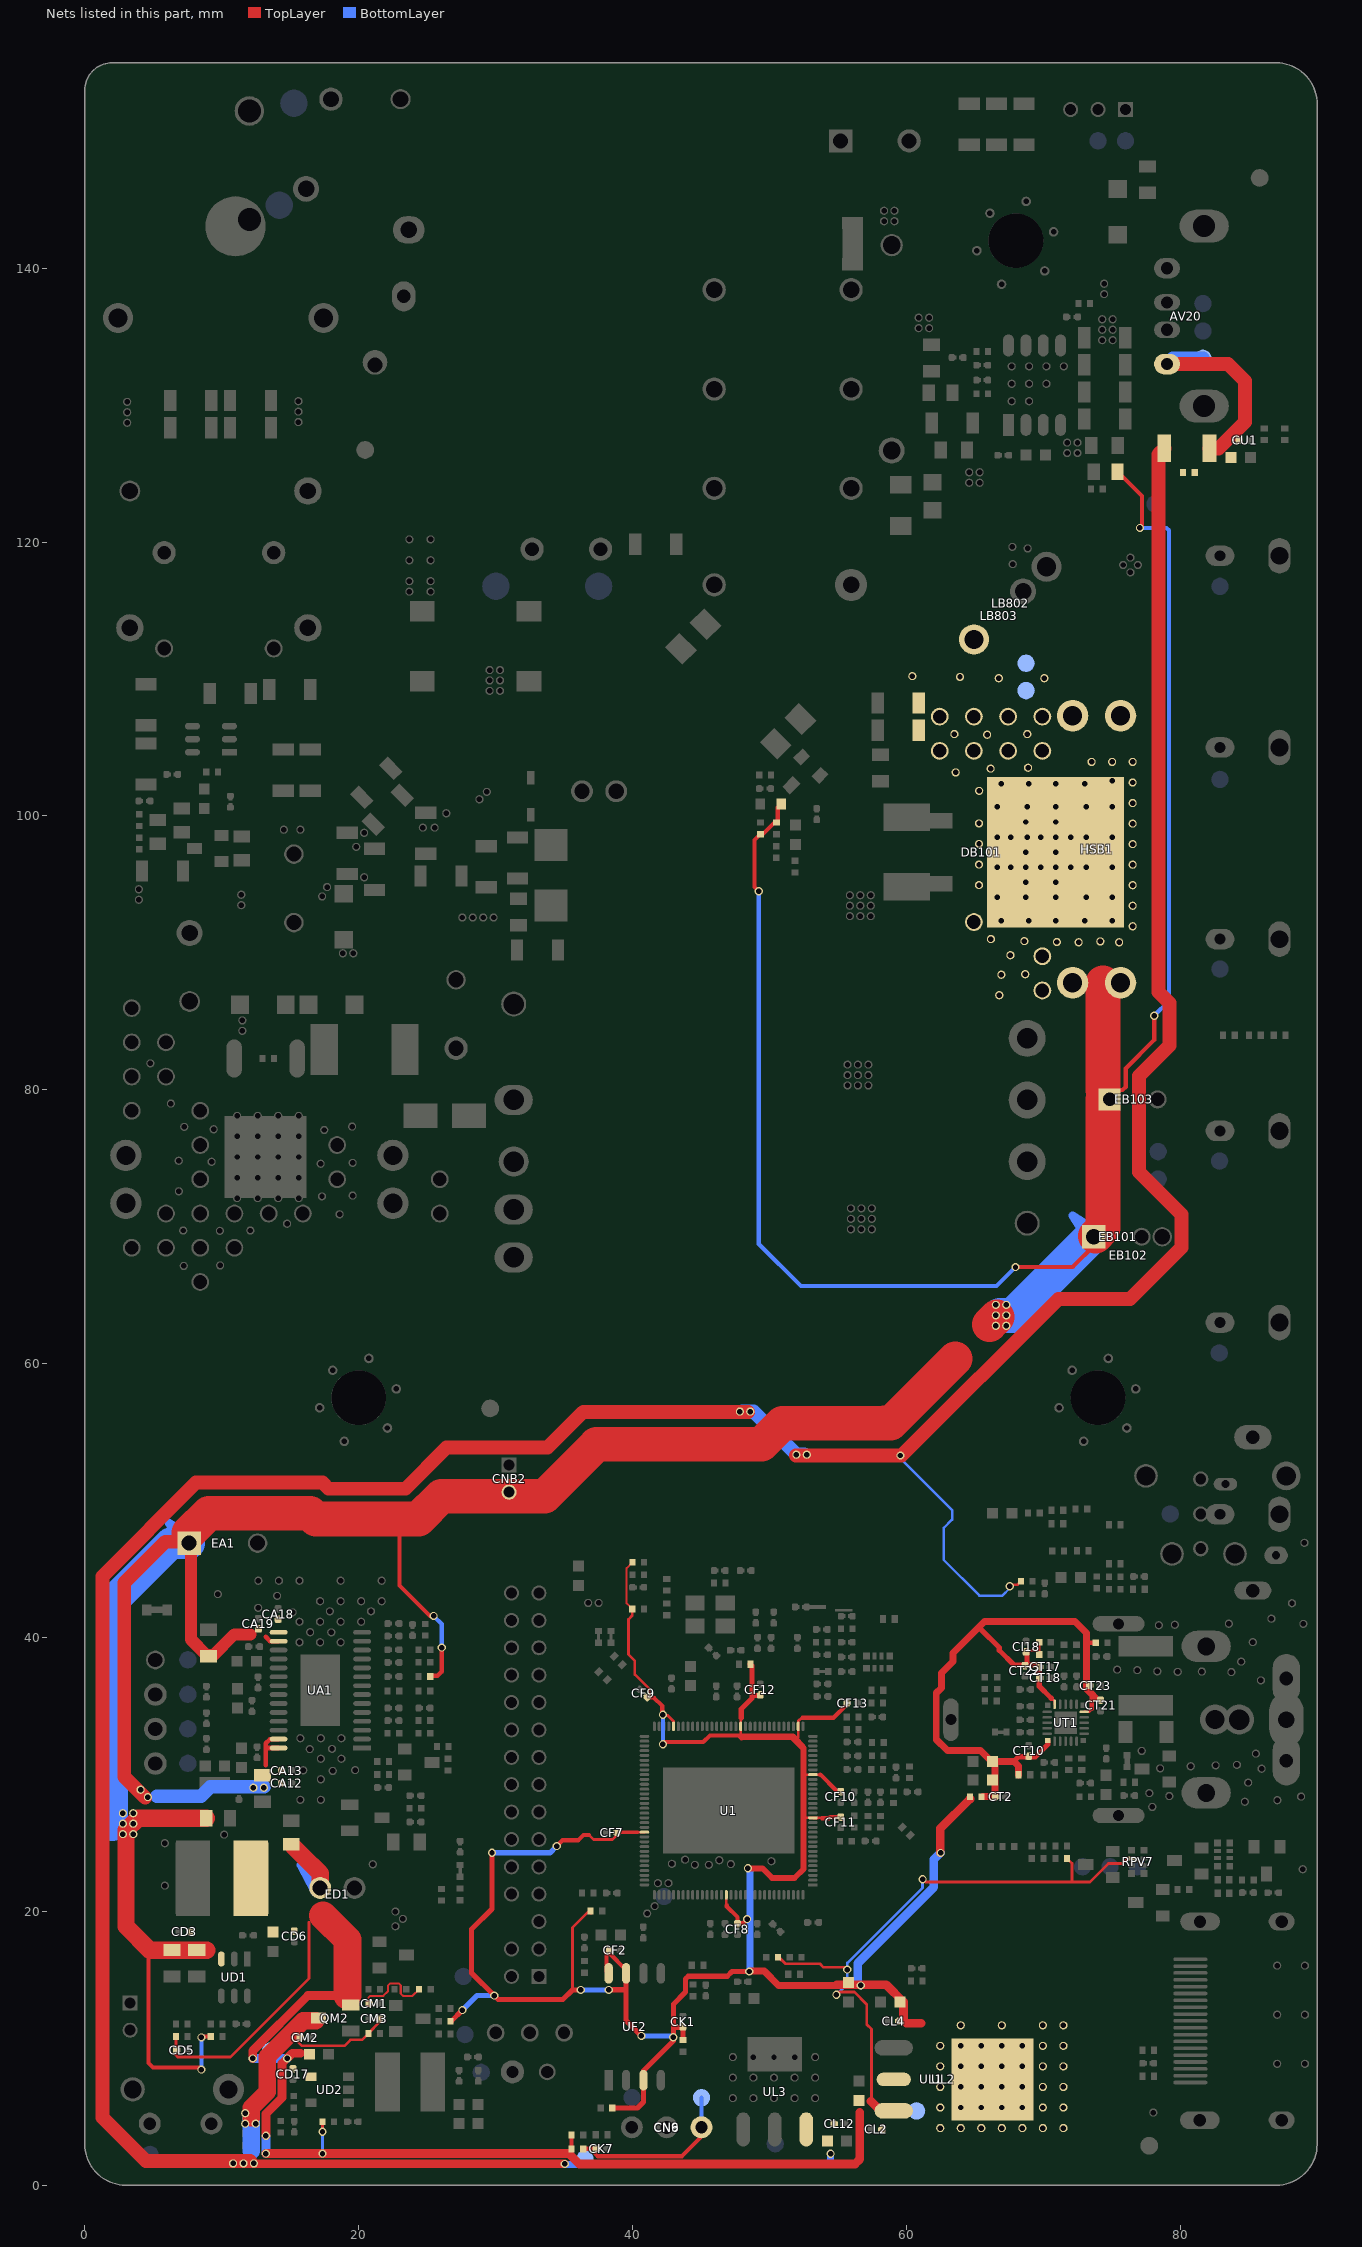
[diagram p0: the nets of this part, all layers, seen from the top]
# Altium PCB MISC116569.PcbDoc (part 6 of 15)
Units mm, origin at the board's own origin, x right, y up, seen from the top; angles counter-clockwise.
Board outline 90 x 155 mm, 2 copper layers (TopLayer, BottomLayer), stack 1.571 mm thick; 527 components, 277 nets, 2450 pads, 649 vias.

## Free pads (board coordinates)
  oval 4x5 on Keep-Out: 0(5,64.09) 0(5,216.893) 0(175.009,93.112) 0(175.009,248.115)
  round 4 on Keep-Out: 0(5,150.003) 0(5,305.005) 0(175.009,5) 0(175.009,160.003)
  round 0.6 hole 0.4 paste-0.4 mask-0.4: VIA5(2.781,25.641) VIA5(2.781,26.403) VIA5(2.781,27.165) VIA5(3.094,128.714) VIA5(3.094,129.476) VIA5(3.094,130.238) VIA5(3.543,25.641) VIA5(3.543,26.403) VIA5(3.543,27.165) VIA5(3.95,93.878) VIA5(3.95,94.64) VIA5(4.071,28.885) VIA5(4.61,28.346) VIA5(4.788,81.928) VIA5(5.85,21.882) VIA5(5.85,24.977) VIA5(6.286,78.994) VIA5(6.858,74.816) VIA5(6.871,72.583) VIA5(7.188,69.723) VIA5(7.226,67.132) VIA5(7.264,77.292) VIA5(9.258,74.739) VIA5(9.411,77.114) VIA5(9.722,43.167) VIA5(9.868,69.698) VIA5(9.881,67.17) VIA5(10.173,25.603) VIA5(10.828,1.587) VIA5(11.126,72.091) VIA5(11.126,73.591) VIA5(11.126,75.091) VIA5(11.126,76.591) VIA5(11.126,78.091) VIA5(11.43,93.485) VIA5(11.43,94.247) VIA5(11.506,84.303) VIA5(11.506,85.065) VIA5(11.59,1.587) VIA5(11.717,4.496) VIA5(11.717,5.258) VIA5(12.09,69.723) VIA5(12.319,29.032) VIA5(12.352,1.587) VIA5(12.479,4.496) VIA5(12.626,72.091) VIA5(12.626,73.591) VIA5(12.626,75.091) VIA5(12.626,76.591) VIA5(12.626,78.091) VIA5(12.662,42.164) VIA5(12.68,44.149) VIA5(13.081,29.032) VIA5(14.046,43.04) VIA5(14.126,72.091) VIA5(14.126,73.591) VIA5(14.126,75.091) VIA5(14.126,76.591) VIA5(14.126,78.091) VIA5(14.18,44.149) VIA5(14.541,98.996) VIA5(14.77,70.218) VIA5(15.173,41.831) VIA5(15.603,128.765) VIA5(15.603,129.527) VIA5(15.603,130.289) VIA5(15.626,72.091) VIA5(15.626,73.591) VIA5(15.626,75.091) VIA5(15.626,76.591) VIA5(15.626,78.091) VIA5(15.68,39.649) VIA5(15.68,41.149) VIA5(15.68,44.149) VIA5(15.743,28.143) VIA5(15.743,32.643) VIA5(15.748,98.996) VIA5(15.951,30.302) VIA5(16.429,31.852) VIA5(16.454,40.386) VIA5(17.18,39.649) VIA5(17.18,41.149) VIA5(17.18,42.649) VIA5(17.221,74.6) VIA5(17.243,28.143) VIA5(17.243,29.643) VIA5(17.243,31.143) VIA5(17.243,32.643) VIA5(17.323,72.212) VIA5(17.332,94.12) VIA5(17.488,77.064) VIA5(17.691,94.805) VIA5(17.902,41.91) VIA5(18.004,40.373) VIA5(18.055,31.864) VIA5(18.105,30.251) VIA5(18.605,70.904) VIA5(18.68,39.649) VIA5(18.68,41.149) VIA5(18.68,42.649) VIA5(18.68,44.149) VIA5(18.743,31.143) VIA5(18.743,32.643) VIA5(18.848,89.967) VIA5(19.52,77.318) VIA5(19.558,72.276) VIA5(19.558,74.663) VIA5(19.61,89.967) VIA5(19.744,30.315) VIA5(19.825,97.739) VIA5(20.18,41.149) VIA5(20.18,42.649) VIA5(20.396,95.517) VIA5(20.396,98.768) VIA5(20.902,41.91) VIA5(21.032,23.437) VIA5(21.68,42.649) VIA5(21.68,44.149) VIA5(22.69,18.91) VIA5(22.69,19.988) VIA5(23.229,19.449) VIA5(23.706,116.383) VIA5(23.706,117.145) VIA5(23.706,118.669) VIA5(23.706,120.193) VIA5(24.689,99.149) VIA5(25.251,116.383) VIA5(25.251,117.145) VIA5(25.251,118.669) VIA5(25.251,120.193) VIA5(25.546,99.149) VIA5(26.403,100.19) VIA5(27.572,92.581) VIA5(28.334,92.581) VIA5(28.824,101.214) VIA5(29.096,92.581) VIA5(29.362,101.752) VIA5(29.561,109.131) VIA5(29.561,109.893) VIA5(29.561,110.655) VIA5(29.858,92.581) VIA5(30.323,109.131) VIA5(30.323,109.893) VIA5(30.323,110.655) VIA5(36.762,42.522) VIA5(37.524,42.522) VIA5(41.07,19.843) VIA5(41.613,20.386) VIA5(41.859,22.06) VIA5(42.626,22.06) VIA5(42.883,23.47) VIA5(43.836,23.774) VIA5(44.559,23.393) VIA5(45.575,23.393) VIA5(46.337,23.736) VIA5(47.188,23.457) VIA5(47.334,6.361) VIA5(47.334,7.861) VIA5(47.334,9.361) VIA5(47.841,56.502) VIA5(48.603,56.502) VIA5(48.834,6.361) VIA5(48.834,7.861) VIA5(48.834,9.361) VIA5(50.147,23.66) VIA5(50.334,6.361) VIA5(50.334,7.861) VIA5(50.334,9.361) VIA5(51.834,6.361) VIA5(51.834,7.861) VIA5(51.834,9.361) VIA5(51.968,53.353) VIA5(52.73,53.353) VIA5(53.334,6.361) VIA5(53.334,7.861) VIA5(53.334,9.361) VIA5(55.702,80.315) VIA5(55.702,81.077) VIA5(55.702,81.839) VIA5(55.875,92.685) VIA5(55.875,93.447) VIA5(55.875,94.209) VIA5(55.956,69.812) VIA5(55.956,70.574) VIA5(55.956,71.336) VIA5(56.464,80.315) VIA5(56.464,81.077) VIA5(56.464,81.839) VIA5(56.637,92.685) VIA5(56.637,93.447) VIA5(56.637,94.209) VIA5(56.718,69.812) VIA5(56.718,70.574) VIA5(56.718,71.336) VIA5(57.226,80.315) VIA5(57.226,81.077) VIA5(57.226,81.839) VIA5(57.399,92.685) VIA5(57.399,93.447) VIA5(57.399,94.209) VIA5(57.48,69.812) VIA5(57.48,70.574) VIA5(57.48,71.336) VIA5(58.369,143.435) VIA5(58.369,144.197) VIA5(59.131,143.435) VIA5(59.131,144.197) VIA5(60.438,110.211) VIA5(60.896,135.623) VIA5(60.896,136.385) VIA5(61.658,135.623) VIA5(61.658,136.385) VIA5(62.473,4.175) VIA5(62.473,5.675) VIA5(62.473,7.175) VIA5(62.473,8.675) VIA5(62.473,10.175) VIA5(63.511,105.981) VIA5(63.602,103.175) VIA5(63.918,110.147) VIA5(63.973,11.675) VIA5(63.973,4.175) VIA5(63.973,5.675) VIA5(63.973,7.175) VIA5(63.973,8.675) VIA5(63.973,10.175) VIA5(64.587,124.333) VIA5(64.587,125.095) VIA5(65.305,99.451) VIA5(65.305,94.951) VIA5(65.305,96.451) VIA5(65.305,97.951) VIA5(65.316,101.829) VIA5(65.349,124.333) VIA5(65.349,125.095) VIA5(65.473,4.175) VIA5(65.473,5.675) VIA5(65.473,7.175) VIA5(65.473,8.675) VIA5(65.473,10.175) VIA5(65.899,105.931) VIA5(66.154,103.454) VIA5(66.18,91.008) VIA5(66.535,62.763) VIA5(66.535,63.525) VIA5(66.535,64.287) VIA5(66.75,110.058) VIA5(66.789,86.906) VIA5(66.942,88.405) VIA5(66.973,11.675) VIA5(66.973,4.175) VIA5(66.973,5.675) VIA5(66.973,7.175) VIA5(66.973,8.675) VIA5(66.973,10.175) VIA5(67.297,62.763) VIA5(67.297,63.525) VIA5(67.297,64.287) VIA5(67.602,89.827) VIA5(67.691,130.289) VIA5(67.691,131.559) VIA5(67.691,132.829) VIA5(67.742,119.647) VIA5(67.767,118.389) VIA5(68.473,4.175) VIA5(68.473,5.675) VIA5(68.473,7.175) VIA5(68.473,8.675) VIA5(68.473,10.175) VIA5(68.618,90.856) VIA5(68.68,88.443) VIA5(68.833,105.981) VIA5(68.859,119.532) VIA5(68.885,103.518) VIA5(68.961,130.289) VIA5(68.961,131.559) VIA5(68.961,132.829) VIA5(69.973,11.675) VIA5(69.973,4.175) VIA5(69.973,5.675) VIA5(69.973,7.175) VIA5(69.973,8.675) VIA5(69.973,10.175) VIA5(70.077,110.058) VIA5(70.231,131.559) VIA5(70.231,132.829) VIA5(70.991,90.792) VIA5(71.473,11.675) VIA5(71.473,4.175) VIA5(71.473,5.675) VIA5(71.473,7.175) VIA5(71.473,8.675) VIA5(71.473,10.175) VIA5(71.501,132.829) VIA5(71.737,126.505) VIA5(71.737,127.267) VIA5(72.499,126.505) VIA5(72.499,127.267) VIA5(72.58,90.771) VIA5(73.523,103.941) VIA5(74.167,90.83) VIA5(74.303,134.747) VIA5(74.303,135.509) VIA5(74.303,136.271) VIA5(74.443,138.108) VIA5(74.443,138.87) VIA5(75.023,103.941) VIA5(75.065,134.747) VIA5(75.065,135.509) VIA5(75.065,136.271) VIA5(75.395,37.655) VIA5(75.54,90.771) VIA5(75.829,118.326) VIA5(76.367,117.787) VIA5(76.367,118.865) VIA5(76.523,103.941) VIA5(76.523,102.441) VIA5(76.523,100.941) VIA5(76.523,99.441) VIA5(76.523,94.941) VIA5(76.523,96.441) VIA5(76.523,97.941) VIA5(76.523,93.441) VIA5(76.523,91.941) VIA5(76.868,37.617) VIA5(76.906,118.326) VIA5(77.186,31.712) VIA5(77.745,28.639) VIA5(77.96,27.622) VIA5(78.037,5.309) VIA5(78.329,37.529) VIA5(78.443,40.894) VIA5(78.532,30.442) VIA5(79.205,28.423) VIA5(79.611,40.932) VIA5(79.815,37.49) VIA5(80.767,30.594) VIA5(81.58,37.516) VIA5(82.583,30.658) VIA5(83.556,41.006) VIA5(83.739,37.478) VIA5(84.145,30.696) VIA5(84.455,38.24) VIA5(84.722,28.003) VIA5(84.963,29.4) VIA5(85.3,39.662) VIA5(85.53,31.521) VIA5(85.898,36.868) VIA5(85.941,30.416) VIA5(86.665,41.375) VIA5(87.079,8.865) VIA5(87.079,12.452) VIA5(87.079,16.04) VIA5(87.097,28.118) VIA5(88.163,42.5) VIA5(88.824,28.384) VIA5(88.946,23.076) VIA5(88.997,40.996) VIA5(89.073,46.914) VIA5(89.111,8.865) VIA5(89.111,12.452) VIA5(89.111,16.04)
  round 1.3 hole 1 paste-0.65 mask-0.051: VIA5(3.427,68.463) VIA5(3.427,78.463) VIA5(3.427,80.963) VIA5(3.427,83.463) VIA5(3.427,85.963) VIA5(5.927,80.963) VIA5(5.927,83.463) VIA5(5.927,68.463) VIA5(5.927,70.963) VIA5(8.427,65.964) VIA5(8.427,68.463) VIA5(8.427,70.963) VIA5(8.427,73.464) VIA5(8.427,75.964) VIA5(8.427,78.464) VIA5(10.927,68.464) VIA5(10.927,70.964) VIA5(13.427,70.964) VIA5(15.927,70.964) VIA5(18.427,73.464) VIA5(18.427,75.964) VIA5(25.927,70.964) VIA5(25.927,73.463) VIA5(62.432,104.752) VIA5(62.432,107.252) VIA5(64.932,92.252) VIA5(64.932,104.752) VIA5(64.932,107.252) VIA5(67.432,104.752) VIA5(67.432,107.252) VIA5(69.932,87.252) VIA5(69.932,89.752) VIA5(69.932,104.752) VIA5(69.932,107.252)

## Via types
v1: diameter 0.6, hole 0.4, TopLayer to BottomLayer, tented both sides, 649 vias

## Nets (pads, with @x,y where several pads share a name; then routed paths per layer and width w, separated by ;. In a path a pad name is that pad's centre, name@x,y a point inside that pad or via, vN(x,y) a via of type N, cw(c..) or ccw(c..) an arc to the next point about the centre after c; other vN are vias at no path point)
3V3_STB: 3V3_STB.1 CF2.2@38.288,17.147 CF2.2@38.463,17.147 CF5.2 CF7.2@38.732,25.745 CF7.2@38.907,25.745 CF8.2@47.666,18.958 CF8.2@47.666,19.133 CF9.2@40.977,35.741 CF9.2@41.101,35.617 CF10.2@55.207,28.78 CF10.2@55.207,28.605 CF11.1 CF12.2@49.335,35.772 CF12.2@49.335,35.947 CF13.2@55.645,35.204 CF13.2@55.821,35.204 CK1.2@43.683,11.511 CK1.2@43.683,11.686 CL3.2 CL4.2@59.319,11.991 CL4.2@59.494,11.991 L3.1 pad.VIA5@62.473,4.175 pad.VIA5@62.473,5.675 pad.VIA5@62.473,7.175 pad.VIA5@62.473,8.675 pad.VIA5@62.473,10.175 pad.VIA5@63.973,4.175 pad.VIA5@63.973,5.675 pad.VIA5@63.973,7.175 pad.VIA5@63.973,8.675 pad.VIA5@63.973,10.175 pad.VIA5@63.973,11.675 pad.VIA5@65.473,4.175 pad.VIA5@65.473,5.675 pad.VIA5@65.473,7.175 pad.VIA5@65.473,8.675 pad.VIA5@65.473,10.175 pad.VIA5@66.973,4.175 pad.VIA5@66.973,5.675 pad.VIA5@66.973,7.175 pad.VIA5@66.973,8.675 pad.VIA5@66.973,10.175 pad.VIA5@66.973,11.675 pad.VIA5@68.473,4.175 pad.VIA5@68.473,5.675 pad.VIA5@68.473,7.175 pad.VIA5@68.473,8.675 pad.VIA5@68.473,10.175 pad.VIA5@69.973,4.175 pad.VIA5@69.973,5.675 pad.VIA5@69.973,7.175 pad.VIA5@69.973,8.675 pad.VIA5@69.973,10.175 pad.VIA5@69.973,11.675 pad.VIA5@71.473,4.175 pad.VIA5@71.473,5.675 pad.VIA5@71.473,7.175 pad.VIA5@71.473,8.675 pad.VIA5@71.473,10.175 pad.VIA5@71.473,11.675 RA35.2 RF3.2 RF29.2 RK4.2 RK13.2 RM1.2 RT1.1 U1.15 U1.24 U1.34 U1.46 U1.60 U1.85 U1.112 UF2.3 UF2.7 UF2.8 UL1.2 UL1.4 UL2.2 | length 177.9
  TopLayer w0.127: RM1.2@39.981,42.078 39.568,42.491 39.568,45.068 RA35.2@39.994,45.494
  TopLayer w0.178: U1.112@46.849,21.207 46.85,20.405 46.881,20.374 46.899,20.356
  TopLayer w0.203: 35.623,14.269 35.623,18.82 36.832,20.03 RF29.2@36.939,20.03 ; 36.861,25.545 37.161,25.245 38.533,25.245 CF7.2@38.883,25.595 ; RF29.2@36.939,19.882 RF29.2@37.008,19.882 ; CF7.2@38.907,25.619 CF7.2@38.907,25.745 CF7.2@38.907,25.758 ; CF7.2@38.907,25.782 CF7.2@38.944,25.782 ; RM1.2@39.981,42.078 39.981,41.609 39.7,41.328 39.7,38.756 40.172,38.285 40.172,37.294 41.231,36.235 41.231,35.747 41.125,35.642 CF9.2@41.101,35.617 ; 40.368,25.782 U1.85@40.873,25.782 ; v1@42.273,34.305 42.578,34.305 42.999,33.884 U1.60@42.999,33.508 ; 47.9,32.78 U1.46@47.9,33.457 ; U1.46@47.899,33.508 47.9,34.127 ; 51.904,32.534 52.1,32.73 U1.34@52.1,33.507 ; U1.34@52.099,33.508 52.099,33.883 52.376,34.16 52.447,34.16 ; 52.494,29.982 U1.24@53.175,29.982 53.716,29.982 ; 52.53,26.832 U1.15@53.175,26.832 ; 53.555,26.821 53.186,26.821 U1.15@53.175,26.832 ; 53.813,26.832 U1.15@53.175,26.832
  TopLayer w0.254: CF7.2@38.907,25.745 38.944,25.782 40.368,25.782
  TopLayer w0.305: v1(34.463,24.767) 34.89,25.194 36.036,25.194 ; 36.062,25.221 36.412,25.571 36.826,25.571 ; UF2.8@38.113,15.619 38.113,16.972 CF2.2@38.276,17.135 ; CF2.2@38.26,17.132 38.276,17.147 CF2.2@38.276,17.135 ; CF2.2@38.288,17.147 CF2.2@38.276,17.135 ; UF2.7@39.53,15.725 38.276,16.98 CF2.2@38.276,17.135 ; CF9.2@41.067,35.642 CF9.2@41.125,35.642 ; CF9.2@41.101,35.617 41.548,35.617 42.177,34.988 v1@42.177,34.352 ; v1@42.375,32.362 45.164,32.362 45.655,32.853 47.754,32.853 47.968,32.64 ; 46.881,20.449 46.881,20.374 46.881,20.359 47.666,19.574 CF8.2@47.666,19.133 48.061,19.133 v1(48.369,19.44) ; 52.425,34.138 53.848,34.138 54.674,34.138 CF13.2@55.652,35.116 ; 53.716,29.982 54.918,28.78 CF10.2@55.207,28.78 ; 53.848,26.797 54.356,26.797 54.438,26.879 CF11.1@55.207,26.879
  TopLayer w0.381: RK13.2@26.703,11.979 26.767,11.979 v1(27.579,12.791) ; v1(29.738,24.272) 29.738,20.183 28.245,18.689 28.245,15.504 v1(29.904,13.845) 30.196,13.553 34.907,13.553 35.619,14.265 v1(36.228,14.265) ; v1@38.267,14.271 39.473,14.271 ; RF3.2@38.526,5.641 40.368,5.641 40.8,6.073 UF2.3@40.8,7.671 40.8,8.36 42.985,10.544 42.985,11.725 ; UF2.7@39.53,15.967 39.53,15.725 UF2.7@39.53,15.471 39.53,12.017 v1(40.648,10.899) ; RK4.2@43.645,10.6 RK4.2@43.683,10.6 CK1.2@43.683,11.511 43.198,11.511 42.985,11.725 ; 47.943,34.127 47.943,34.774 48.732,35.563 48.732,36.426 ; v1(48.527,15.608) 47.269,15.608 46.924,15.263 44.072,15.263 43.878,15.069 43.878,14.103 42.985,13.21 42.985,11.725 ; L3.1@48.578,38.052 L3.1@48.615,38.015 ; L3.1@48.616,38.052 48.732,37.936 48.732,36.426 ; 48.732,35.792 48.732,36.426 ; 48.752,35.772 CF12.2@49.335,35.772
  TopLayer w0.432: v1@48.45,23.137 49.492,23.137 50.196,22.433 51.829,22.433 52.494,23.098 52.494,29.982 52.494,31.944
  TopLayer w0.508: 48.08,32.752 51.686,32.752 51.904,32.534 52.394,32.044 ; v1@48.573,15.654 49.622,15.654 50.676,14.6 54.923,14.6 ; v1@62.476,24.3 62.476,24.29 v1(62.497,24.27)
  TopLayer w0.635: 54.923,14.632 CF5.2@55.761,14.632 ; CF5.2@55.761,14.806 55.935,14.632 58.532,14.632 59.788,13.376 59.788,12.053 60.015,11.826 61.095,11.826 ; v1@62.485,24.3 62.485,26.046 RT1.1@64.645,28.206
  BottomLayer w0.305: v1(42.223,32.21) v1(42.222,34.352)
  BottomLayer w0.381: v1(27.579,12.791) 28.634,13.845 v1(29.904,13.845) ; v1(29.738,24.272) 33.968,24.272 v1(34.463,24.767) ; v1(36.228,14.265) v1(38.26,14.265) ; v1(40.648,10.899) v1@42.893,10.899
  BottomLayer w0.508: v1@48.573,15.654 v1@48.573,23.015
  BottomLayer w0.635: 56.443,15.021 56.443,16.199 ; v1(56.667,14.592) 56.443,14.817 56.443,16.199 ; v1(62.497,24.27) 62.009,23.782 62.009,21.765 56.443,16.199
  other v1: 42.981,10.811 48.433,23.155
3V3_TUN: CI18.2@68.745,38.907 CI18.2@68.745,39.082 CT1.2 CT2.2@66.47,28.362 CT2.2@66.645,28.362 CT10.2@68.943,31.289 CT10.2@68.943,31.464 CT17.1 CT18.2@69.708,37.046 CT18.2@69.883,37.046 CT21.2@74.181,35.46 CT21.2@74.181,35.285 CT22.1 CT23.1 CT52.2 FT2.2 RF43.1 RF44.1 RT1.2 RT5.1 UT1.6 UT1.12 UT1.19 | length 56
  TopLayer w0.178: 70.635,35.547 70.832,35.351 UT1.12@70.832,35.122 ; UT1.6@72.982,34.572 73.338,34.572 73.546,34.78
  TopLayer w0.203: CI18.2@68.819,39.027 69.634,39.027 ; RF43.1@69.699,38.776 RF44.1@69.699,39.652 RF44.1@69.699,39.677
  TopLayer w0.305: CT17.1@69.687,37.645 69.687,37.036 69.687,36.467 69.708,36.446 70.607,35.547 ; 73.307,39.611 RT5.1@73.832,39.611 ; 73.546,34.78 73.546,35.855
  TopLayer w0.381: 65.425,40.631 66.784,39.271 ; 66.789,39.266 66.784,39.271 ; 67.851,30.952 68.188,31.289 69.42,31.289 70.337,32.206 UT1.19@70.337,32.477 ; CT22.1@68.687,38.013 CT17.1@69.525,38.013 ; CT22.1@68.819,38.145 CI18.2@68.819,39.027 ; CT17.1@69.568,38.013 69.708,37.874 69.708,36.446 ; 69.683,36.453 70.576,35.559 ; CT18.2@69.687,37.036 CT17.1@69.687,37.852 ; CT17.1@69.708,37.848 69.567,37.99 CT22.1@68.664,37.99 67.86,37.99 66.784,39.065 66.784,39.271
  TopLayer w0.508: 62.183,35.445 62.183,34.938 ; 64.028,31.74 64.435,31.74 ; RT1.2@65.578,28.374 66.457,28.374 66.457,30.784 CT52.2@66.289,30.952 ; FT2.2@68.195,29.962 68.195,30.609 67.851,30.952 66.215,30.952 65.428,31.74 64.435,31.74 ; 73.789,35.611 73.546,35.855 73.142,36.258 73.142,40.342 72.307,41.178 65.713,41.178 63.401,38.867 63.401,38.261 62.563,37.423 62.563,36.32 62.183,35.94 62.183,34.938 ; 62.183,34.938 62.183,32.555 62.998,31.74 64.435,31.74
5V_IR: 5V_IR.1 CK7.1 CN6.3 CN9.3 RK18.1 | length 12.6
  TopLayer w0.305: RK18.1@36.406,2.657 CK7.1@37.306,2.657 37.306,2.278 37.463,2.121 38.641,2.121 ; 38.566,2.121 38.641,2.121 ; CN9.3@45.034,4.227 45.034,3.548 43.607,2.121 38.641,2.121
  BottomLayer w0.305: CN9.3@45.042,4.234 5V_IR.1@45.042,6.391
5V_M: 5V_M.1 CL11.2 CL12.2@54.682,4.486 CL12.2@54.857,4.486 CM2.2@15.686,10.782 CM2.2@15.861,10.782 CM3.1 FU1.2 pad.VIA5@10.828,1.587 pad.VIA5@11.59,1.587 pad.VIA5@11.717,4.496 pad.VIA5@11.717,5.258 pad.VIA5@12.352,1.587 pad.VIA5@12.479,4.496 pad.VIA5@47.841,56.502 pad.VIA5@48.603,56.502 pad.VIA5@51.968,53.353 pad.VIA5@52.73,53.353 QM2.D RK10.2 RO2.1 RU4.2 UL3.3 | length 287.8
  TopLayer w0.178: v1(67.55,43.738) 67.674,43.862 68.12,43.862 RO2.1@68.365,44.107
  TopLayer w0.203: 15.038,11.005 15.864,10.179 18.953,10.179 19.391,10.617 20.237,10.617 RK10.2@20.71,11.09 20.71,11.101 21.559,11.95 CM3.1@21.559,12.141 ; QM2.D@16.962,12.097 QM2.D@17.07,12.205
  TopLayer w0.61: 12.086,1.765 12.289,1.562 v1@35.044,1.562
  TopLayer w1.016: 1.283,17.729 1.283,16.777 ; 12.086,1.765 4.453,1.765 1.283,4.935 1.283,16.777 ; pad.VIA5@48.435,56.477 36.402,56.477 33.796,53.871 26.423,53.871 23.416,50.863 17.793,50.863 17.348,51.308 8.122,51.308 1.283,44.468 1.283,16.777 ; pad.VIA5@51.93,53.291 56.528,53.291 ; 55.626,53.291 56.528,53.291 ; FU1.2@78.838,126.848 78.405,126.415 78.405,87.147 79.205,86.347 79.205,83.248 76.977,81.021 76.977,73.988 80.086,70.879 80.086,68.495 76.323,64.732 71.1,64.732 59.659,53.291 v1(59.57,53.291) 56.528,53.291
  TopLayer w1.27: 12.149,4.94 12.149,5.664 13.317,6.833 ; 13.317,7.734 13.317,6.833 ; QM2.D@16.879,12.014 15.959,12.014 13.317,9.373 13.317,6.833
  BottomLayer w0.178: v1(59.57,53.291) 59.57,53.079 63.338,49.311 63.338,48.61 62.728,48 62.728,45.661 65.329,43.06 67.012,43.06 67.55,43.598 v1(67.55,43.738)
  BottomLayer w0.508: v1@35.102,1.511 54.184,1.511 54.465,1.793 v1(54.465,2.301)
  BottomLayer w1.016: pad.VIA5@48.019,56.502 pad.VIA5@48.603,56.502 48.843,56.502 51.992,53.353 pad.VIA5@52.514,53.353
  BottomLayer w1.27: 12.149,2.499 12.149,4.889
  other v1: 35.056,1.557
5V_STB: 5V_STB.1 CD5.2@6.663,9.868 CD5.2@6.838,9.868 CD6.2@15.299,18.424 CD6.2@15.299,18.599 CD7.2 CD16.2 CD17.2@15.197,8.368 CD17.2@15.197,8.543 CL1.2 CL2.2@58.068,4.079 CL2.2@58.243,4.079 CM1.2@20.709,13.266 CM1.2@20.884,13.266 ED1.1 LD1.2 LD3.1 QM2.S R5V.1 RD3.2 RD7.2 RF8.2 RF9.2 RK12.2 RK18.2 RM3.2 RPV7.3 UD2.4 UL1.3 UL2.3 | length 150.9
  TopLayer w0.152: 20.709,13.679 20.861,13.83 21.806,13.83 22.157,14.181 22.157,14.593 22.304,14.741 22.929,14.741 23.077,14.592 23.077,13.989 23.249,13.818 23.922,13.818 RM3.2@24.417,14.313
  TopLayer w0.203: RD3.2@6.651,10.858 6.651,9.868 6.651,9.499 6.79,9.36 10.647,9.36 16.383,15.096 16.383,19.202 ; RD7.2@17.357,4.638 17.357,3.903 v1(17.361,3.899) ; RF9.2@50.623,16.652 50.683,16.652 51.161,16.174 52.732,16.174 53.691,16.174 53.951,15.913 55.639,15.913 55.689,15.862 v1(55.689,15.748) ; v1@55.099,14.111 56.206,14.111 57.102,13.215 57.102,11.757 57.453,11.407 57.453,6.18 ; v1@61.389,22.151 73.415,22.151 74.752,23.489 75.782,23.489 76.151,23.858 RPV7.3@76.451,23.858 ; RF8.2@71.742,23.863 72.098,23.508 72.098,22.177
  TopLayer w0.305: RK18.2@35.556,2.657 RK12.2@35.556,3.673
  TopLayer w0.635: v1(12.263,9.258) 12.263,9.809 16.306,13.852 19.187,13.852 ; v1(13.229,2.311) v1(17.361,2.311) 35.354,2.311 36.116,1.549 56.254,1.549 56.599,1.895 56.599,5.309 ; v1(13.229,3.607) 13.229,5.217 14.397,6.386 14.397,8.89 15.146,9.639 15.781,9.639 ; 57.411,6.138 58.12,5.428 UL1.3@59.08,5.428
  TopLayer w1.27: R5V.1@15.297,24.662 15.88,24.079 17.193,22.767 ED1.1@17.193,21.707
  TopLayer w2.032: 17.406,19.705 19.187,17.924 19.187,13.852
  BottomLayer w0.203: v1(17.361,2.311) v1(17.361,3.899) 17.361,3.011 ; v1(54.897,13.909) 55.689,14.701 v1(55.689,15.748) 55.689,16.218 61.189,21.717 v1(61.189,22.352)
  BottomLayer w0.635: v1(12.263,9.258) v1(14.778,9.258) ; v1(13.229,2.311) v1(13.229,3.607)
5V_USB2.0: 5V.1 AV20.1@79.04,133 CU1.1 CU2.1 FU1.1 RU4.1 | length 15.4
  TopLayer w1.016: AV20.1@79.04,133 83.479,133 84.717,131.762 84.717,128.753 82.812,126.848 FU1.1@82.138,126.848
  BottomLayer w1.016: AV20.1@79.04,133 79.457,133.417 5V.1@81.656,133.417
12V: CA1.2 CA2.2 CA12.2@14.327,29.357 CA12.2@14.502,29.358 CA13.2@14.327,30.274 CA13.2@14.502,30.274 CA18.2@14.122,41.29 CA18.2@14.122,41.465 CA19.2@12.675,40.576 CA19.2@12.675,40.752 CD1.1 CD2.1 CD3.2@7.526,18.504 CD3.2@7.701,18.504 CNB2.2 DB101.2 EA1.1 EB101.1@73.687,69.266 EB102.1@73.687,69.266 EB103.1@74.849,79.299 HSB1.1 HSB1.2 HSB1.3 HSB1.4 LB802.1@64.94,112.893 LB803.1 pad.VIA5@2.781,25.641 pad.VIA5@2.781,26.403 pad.VIA5@2.781,27.165 pad.VIA5@3.543,25.641 pad.VIA5@3.543,26.403 pad.VIA5@3.543,27.165 pad.VIA5@4.61,28.346 pad.VIA5@4.071,28.885 pad.VIA5@12.319,29.032 pad.VIA5@13.081,29.032 pad.VIA5@60.438,110.211 pad.VIA5@62.432,104.752 pad.VIA5@62.432,107.252 pad.VIA5@63.511,105.981 pad.VIA5@63.602,103.175 pad.VIA5@63.918,110.147 pad.VIA5@64.932,92.252 pad.VIA5@64.932,104.752 pad.VIA5@64.932,107.252 pad.VIA5@65.305,94.951 pad.VIA5@65.305,96.451 pad.VIA5@65.305,97.951 pad.VIA5@65.305,99.451 pad.VIA5@65.316,101.829 pad.VIA5@65.899,105.931 pad.VIA5@66.18,91.008 pad.VIA5@66.75,110.058 pad.VIA5@66.154,103.454 pad.VIA5@66.535,62.763 pad.VIA5@66.535,63.525 pad.VIA5@66.535,64.287 pad.VIA5@66.789,86.906 pad.VIA5@66.942,88.405 pad.VIA5@67.297,62.763 pad.VIA5@67.297,63.525 pad.VIA5@67.297,64.287 pad.VIA5@67.432,104.752 pad.VIA5@67.432,107.252 pad.VIA5@67.602,89.827 pad.VIA5@68.68,88.443 pad.VIA5@68.618,90.856 pad.VIA5@68.833,105.981 pad.VIA5@68.885,103.518 pad.VIA5@69.932,87.252 pad.VIA5@69.932,89.752 pad.VIA5@69.932,104.752 pad.VIA5@69.932,107.252 pad.VIA5@70.077,110.058 pad.VIA5@70.991,90.792 pad.VIA5@72.58,90.771 pad.VIA5@73.523,103.941 pad.VIA5@74.167,90.83 pad.VIA5@75.023,103.941 pad.VIA5@75.54,90.771 pad.VIA5@76.523,91.941 pad.VIA5@76.523,93.441 pad.VIA5@76.523,94.941 pad.VIA5@76.523,96.441 pad.VIA5@76.523,97.941 pad.VIA5@76.523,99.441 pad.VIA5@76.523,100.941 pad.VIA5@76.523,102.441 pad.VIA5@76.523,103.941 R12V.1 RA25.2 RB123.2 RB124.2 RB131.2 RB135.1 RB158.2 RB816.1 RD1.1 TP_12VA+.1 TP_12VB+.1 UA1.15 UA1.16 UA1.27 UA1.28 UD1.3 | length 321.3
  TopLayer w0.3: v1(49.22,94.501) 48.92,94.801 48.92,98.24 RB158.2@49.347,98.667 ; RB158.2@49.541,98.667 RB135.1@50.453,99.579 ; RB135.1@50.516,99.517 50.606,99.607 50.606,100.616 RB131.2@50.853,100.863 ; v1(67.97,67.056) 72.149,67.056 73.812,68.72 EB101.1@73.812,69.329 ; EB103.1@74.366,79.972 75.781,79.972 76.022,80.213 76.022,81.547 78.1,83.625 v1(78.1,85.407) ; RB816.1@75.423,125.146 77.214,123.355 v1@77.214,121.186
  TopLayer w0.305: 4.643,17.107 4.643,8.928 4.974,8.598 v1@8.364,8.598 ; v1@8.58,10.859 RD1.1@9.204,10.859 ; 22.979,47.625 22.979,43.809 v1@25.213,41.575 ; RA25.2@25.229,37.205 25.77,37.205 26.068,37.503 v1(26.068,39.268)
  TopLayer w0.33: 13.208,40.043 13.522,39.729 UA1.16@14.154,39.729 ; 13.212,30.654 13.212,32.268 13.523,32.579 UA1.27@14.154,32.579 ; 13.264,31.929 UA1.28@14.154,31.929
  TopLayer w0.889: EA1.1@7.544,47.003 7.757,46.79 7.757,39.846 8.875,38.729 9.423,38.729 10.924,40.23 12.078,40.23 ; EA1.1@7.599,47.003 EA1.1@7.72,46.882
  TopLayer w1: pad.VIA5@4.409,28.304 2.875,29.837 2.875,43.989 5.889,47.003 7.544,47.003 7.599,47.003 EA1.1@7.646,47.003
  TopLayer w1.27: CD2.1@5.986,17.173 CD2.1@6.365,17.173 ; R12V.1@8.872,26.81 3.899,26.81 3.01,25.921 3.01,18.905 4.742,17.173 CD2.1@6.365,17.173 ; 8.916,17.173 CD1.1@8.174,17.173 CD2.1@6.365,17.173
  TopLayer w2.54: EA1.1@7.599,47.623 9.048,49.073 16.458,49.073 16.877,48.654 24.367,48.654 26.033,50.32 33.585,50.32 37.38,54.115 49.414,54.115 50.952,55.653 58.405,55.653 ; 58.412,55.66 58.405,55.653 ; 58.592,55.653 58.405,55.653 ; 63.567,60.36 58.86,55.653 58.405,55.653 ; 66.063,62.855 pad.VIA5@66.611,63.404 ; EB101.1@73.812,69.329 74.366,69.883 EB103.1@74.366,79.299 ; EB103.1@74.366,79.972 74.366,87.82
  BottomLayer w0.3: v1(49.22,94.501) 49.22,68.745 52.301,65.664 66.578,65.664 v1(67.97,67.056) ; v1(77.059,121.031) 79.002,121.031 79.17,120.863 79.17,86.477 v1(78.1,85.407)
  BottomLayer w0.305: v1(8.517,8.445) v1(8.517,10.795) ; v1(25.468,41.575) 26.068,40.975 v1(26.068,39.268)
  BottomLayer w1: 5.271,28.402 8.484,28.402 9.177,29.096 12.319,29.096 pad.VIA5@13.081,29.096
  BottomLayer w2.286: 2.014,26.294 2.014,31.001 ; 2.014,29.456 2.014,31.001 ; EA1.1@7.623,46.888 7.039,46.888 6.287,46.888 2.014,42.616 2.014,31.001
  BottomLayer w2.54: pad.VIA5@66.815,63.525 67.789,63.525 EB101.1@73.268,69.004
  other v1: 66.921,92.357 68.921,92.357 70.921,92.357 73.021,92.357 75.021,92.357 66.621,94.057 68.721,94.057 70.921,94.057 73.121,94.057 75.021,94.057 68.721,95.157 70.921,95.157 66.621,96.257 67.621,96.257 68.721,96.257 69.821,96.257 70.921,96.257 72.021,96.257 73.121,96.257 75.021,96.257 68.721,97.357 70.921,97.357 66.621,98.457 67.621,98.457 68.821,98.457 69.821,98.457 70.921,98.457 72.021,98.457 73.121,98.457 75.021,98.457 68.721,99.557 70.921,99.557 66.621,100.657 68.821,100.657 70.921,100.657 73.121,100.657 75.021,100.657 66.921,102.357 68.921,102.357 70.921,102.357 73.021,102.357 75.021,102.557